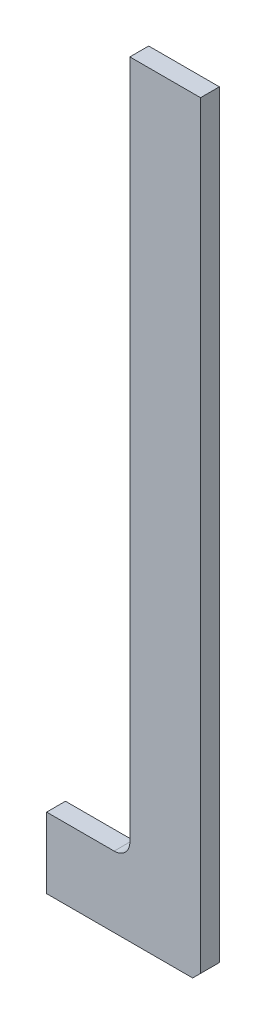
from build123d import *

# Parameters (mm, degrees)
SKETCH_1_W          = 98
SKETCH_1_H          = 488
EXTRUDE_1_DEPTH     = 6
CUT_EXTRUDE_1_REACH = 251.161
SKETCH_2_W          = 53
SKETCH_2_H          = 443
FILLET_1_R          = 10
CHAMFER_1_SIZE      = 5


with BuildPart() as part:
    # 草图1 → 凸台-拉伸1 (new, symmetric)
    with BuildSketch(Plane.XY):
        Rectangle(SKETCH_1_W, SKETCH_1_H)
    extrude(amount=EXTRUDE_1_DEPTH, both=True)

    # 草图2 → 切除-拉伸1 (cut, up to next)
    with BuildSketch(Plane.XY.offset(6), mode=Mode.PRIVATE) as cut_extrude_1_sk1:
        with Locations((-22.5, 22.5)):
            Rectangle(SKETCH_2_W, SKETCH_2_H)
    cut_extrude_1_tool1 = extrude(cut_extrude_1_sk1.sketch, amount=-CUT_EXTRUDE_1_REACH, mode=Mode.PRIVATE) & part.part
    add(cut_extrude_1_tool1.solids().sort_by_distance((-22.5, 22.5, 6))[0], mode=Mode.SUBTRACT)

    # 圆角1
    fillet_1_edges = [part.edges().sort_by_distance(p)[0] for p in [
        (4, -199, 0),
    ]]
    fillet(fillet_1_edges, radius=FILLET_1_R)

    # 倒角1
    chamfer_1_edges = [part.edges().sort_by_distance(p)[0] for p in [
        (49, -244, 0),
    ]]
    chamfer(chamfer_1_edges, length=CHAMFER_1_SIZE)


solid = part.part
